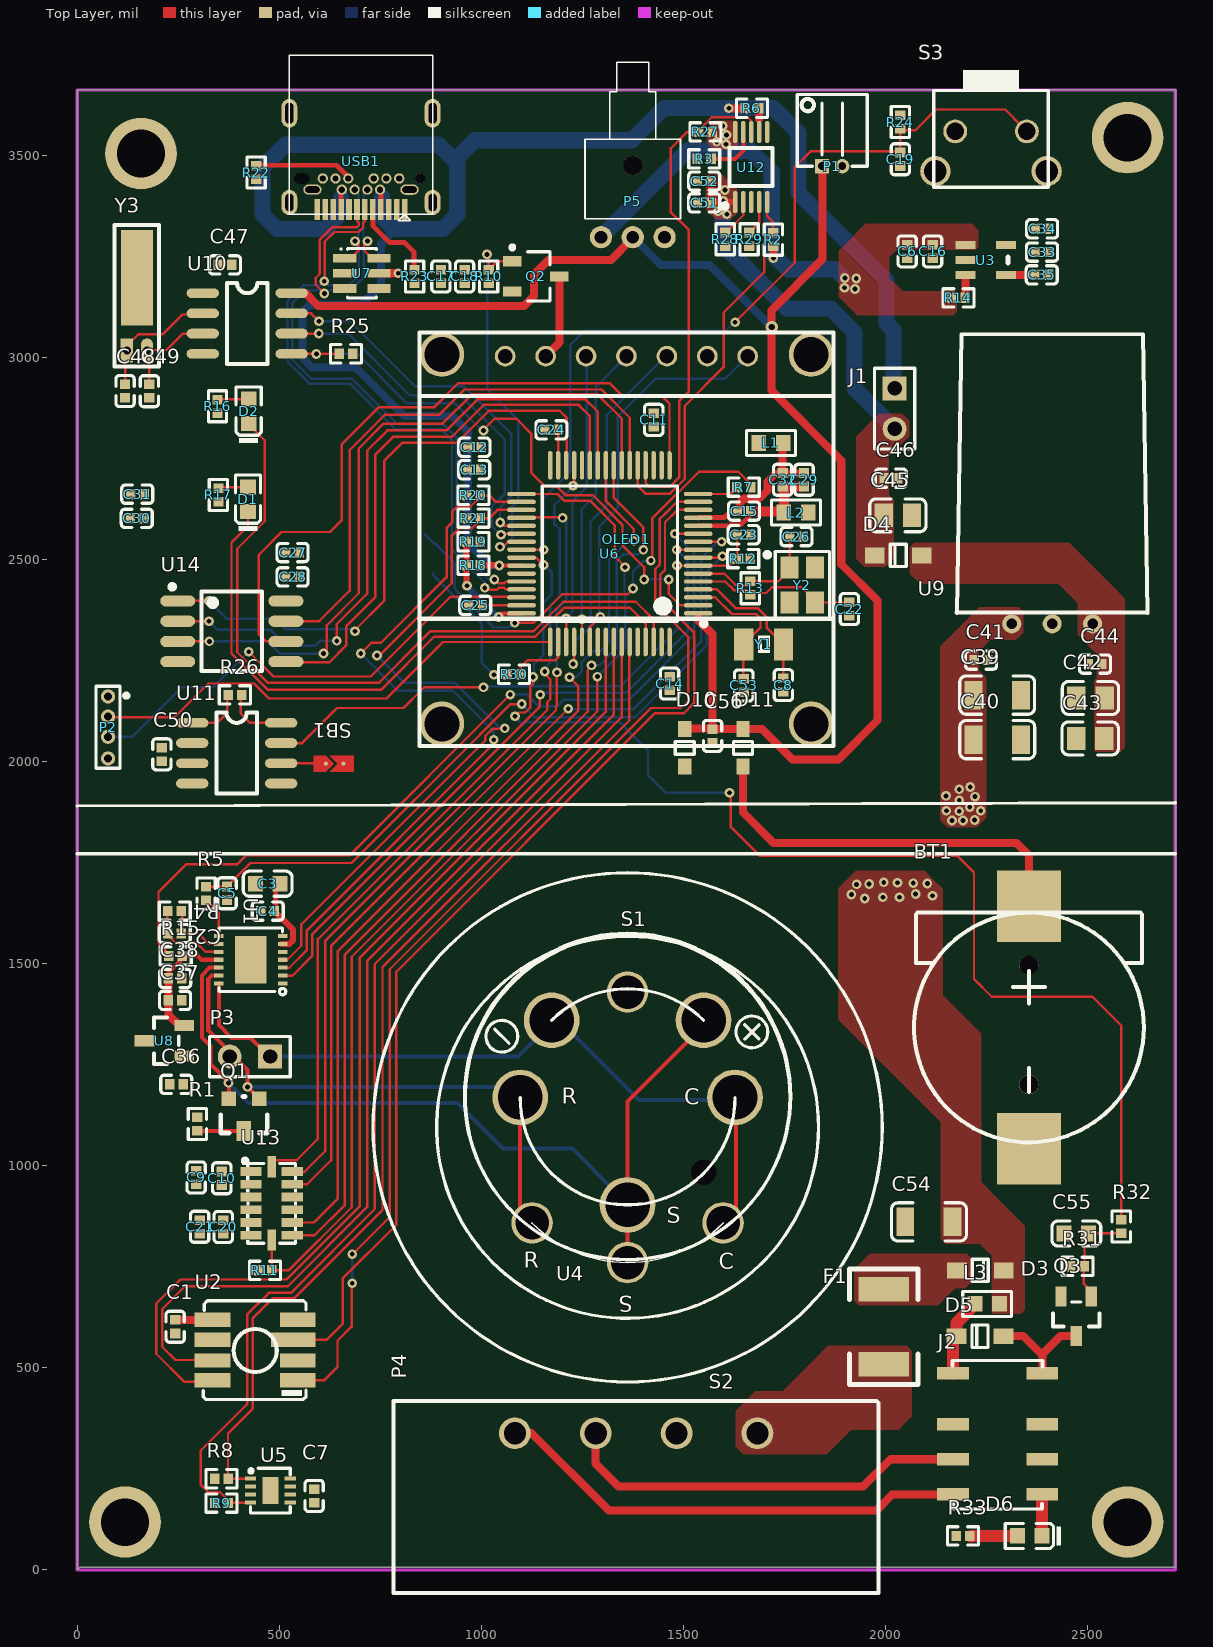
[diagram p0: Top Layer view]
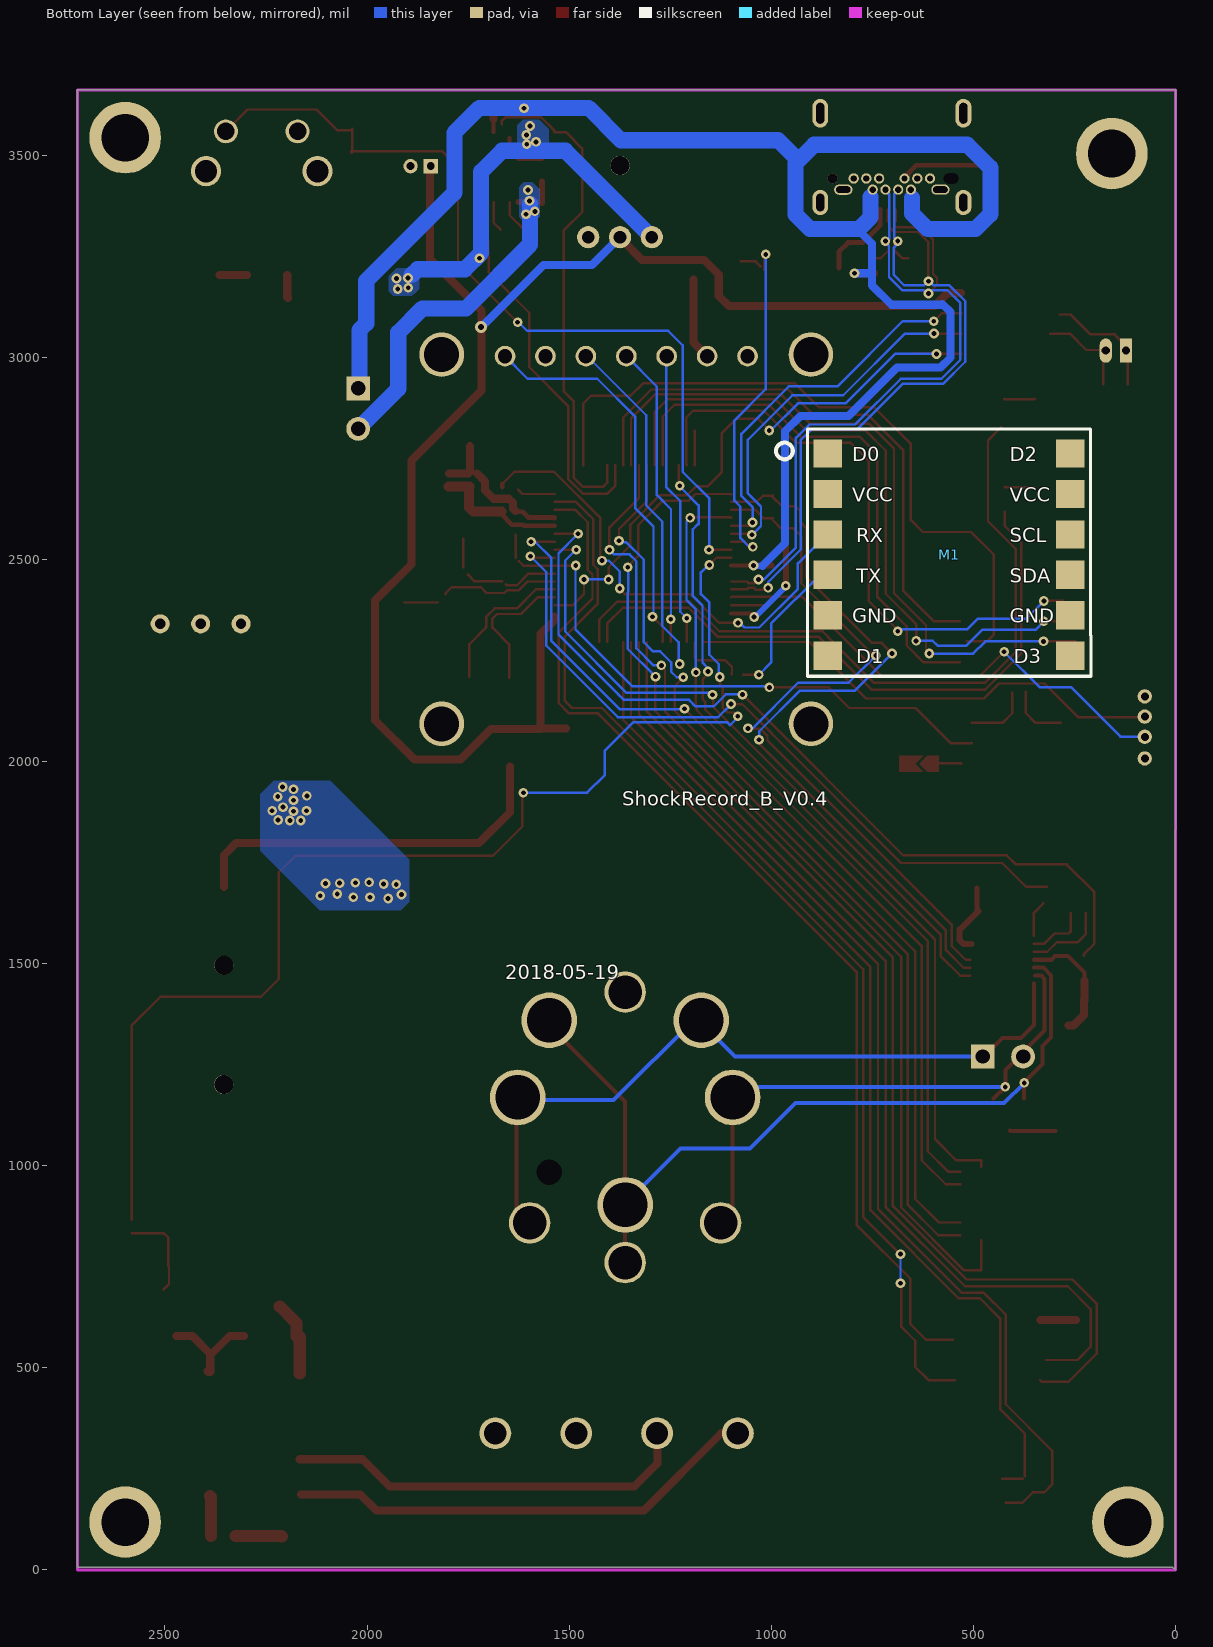
[diagram p1: Bottom Layer view, seen from below]
# Altium PCB MISC105202.PcbDoc (part 1 of 3)
Units mil, origin at the board's own origin, x right, y up, seen from the top; angles counter-clockwise.
Board outline 2717.72 x 3662.2 mil, 4 copper layers (Top Layer, GND, POWER, Bottom Layer), stack 38.217 mil thick; 136 components, 101 nets, 484 pads, 108 vias.
Unrouted connection lines stored in the file: 61.

## Layer stack, top to bottom
Top Layer: signal copper 1.4
Dielectric: core 10, FR-4, Dk 4.2
GND: plane copper 1.417, net GND
Dielectric: prepreg 10, Dk 4.2
POWER: plane copper 1.4, net (Multiple Nets)
Dielectric: core 12.6, FR-4, Dk 4.8
Bottom Layer: signal copper 1.4

## Board outline
0,-0.39 7.09,6.69 2717.32,6.69 2717.32,3661.81 -0.39,3661.81

## Design rules (kind name [scope] priority, off if disabled: settings)
Clearance Clearance_1 [inpolygon] p1: gap=6
Clearance [All] p2: gap=6
DiffPairsRouting [All] p1: maxlimit=6 minlimit=6 mostfreqgap=6 maxuncoupledlength=500
HoleSize [All] p1: absolutevalues=TRUE maxlimit=150 minlimit=10 maxpercent=80.000 minpercent=20.000
MinimumSolderMaskSliver [All] p1: minsoldermaskwidth=0
PlaneClearance [All] p1: clearance=20
PlaneConnect [All] p1: planeconnectstyle=Direct reliefexpansion=20 reliefentries=4 reliefconductorwidth=10 reliefairgap=10
PolygonConnect PolygonConnect_2 [All vs isvia] p1: connectstyle=Direct reliefconductorwidth=10 reliefentries=4 polygonreliefangle="90 Angle"
PolygonConnect PolygonConnect_1 [InNet(gnd)] p2: connectstyle=Relief reliefconductorwidth=15 reliefentries=4 polygonreliefangle="90 Angle"
PolygonConnect [All] p3: connectstyle=Direct reliefconductorwidth=15 reliefentries=4 polygonreliefangle="90 Angle"
RoutingVias [All] p1: holewidth=28 width=50 viastyle="Through Hole" minholewidth=10 minwidth=20 maxholewidth=50 maxwidth=100
SilkToSilkClearance [All] p1: silktosilkclearance=0
SilkscreenOverComponentPads SilkToSolderMaskClearance [IsPad] p1: minsilkscreentomaskgap=0
SolderMaskExpansion [All] p1: expansion=4
Width [All] p1: maxlimit=40 minlimit=6 preferedwidth=6 minimp=50.000000 maximp=50.000000 favimp=50.000000
21 further rules are at their usual default settings.

## Classes and differential pairs
component class ShockRecord_V0.45: C8 C9 C10 C11 C12 C13 C14 C15 C17 C18 C19 C20 C21 C22 C23 C24 C25 C26 C27 C28 C30 C31 C47 C48 C49 C50 C51 C52 C53 D1 D2 M1 OLED1 P1 P2 P5 Q2 R2 R3 R6 R7 R10 R11 R12 R13 R16 R17 R18 R19 R20 R21 R22 R23 R24 R25 R26 R27 R28 R29 R30 S3 SB1 U6 U7 U10 U11 U12 U13 U14 USB1 Y1 Y2 Y3
component class ShockRecord_PWR_V0.45: BT1 C6 C16 C29 C32 C33 C34 C35 C36 C37 C38 C39 C40 C41 C42 C43 C44 C45 C46 C54 C55 C56 D3 D4 D5 D6 D10 D11 F1 J1 J2 L1 L2 L3 P4 Q3 R14 R15 R31 R32 R33 U3 U8 U9
component class ShockRecord_Sensor_V0.45: C1 C2 C3 C4 C5 C7 P3 Q1 R1 R4 R5 R8 R9 S1 S2 U1 U2 U4 U5
differential pair D: +D_P -D_N

## Components (designator, comment, footprint, x,y, rotation, side; value= is the part's Value field where it differs from the comment)
BT1 "CR2032-3V" BT1 2342.52,1322.44 r90 top
C1 "0.1uF,25V" 0402_C 242.13,601.57 r270 top
C2 "1uF (105) 10% 50V" 0402_C 240.94,1574.41 r180 top
C3 "10uF" 0603_C 470.87,1697.64 r0 top
C4 "0.1uF,25V" 0402_C 471,1630 r0 top
C5 "1uF,25V" 0402_C 370.47,1674.02 r90 top
C6 "0.1uF" 0402_C 2053,3262 r270 top
C7 "0.1uF" 0402_C 586,183 r270 top
C8 "2.7pF" 0402_C 1746.85,2188.98 r270 top
C9 "1uF" 0402_C 294.09,970.87 r270 top
C10 "0.1uF" 0402_C 357.48,968.9 r90 top
C11 "0.1uF" 0402_C 1425.98,2845.28 r270 top
C12 "0.1uF" 0402_C 982.28,2777.56 r0 top
C13 "0.1uF" 0402_C 981.89,2721.65 r0 top
C14 "0.1uF" 0402_C 1465.35,2192.91 r90 top
C15 "0.1uF" 0402_C 1649.61,2619.68 r180 top
C16 "10uF" 0402_C 2116,3262 r90 top
C17 "0.1uF" 0402_C 899.61,3200 r270 top
C18 "10uF" 0402_C 958.27,3200 r270 top
C19 "10nF" 0402_C 2036.22,3489.96 r270 top
C20 "1uF" 0402_C 361.02,848.43 r90 top
C21 "0.1uF" 0402_C 302.76,848.82 r270 top
C22 "20pF" 0402_C 1910,2377 r90 top
C23 "0.1uF" 0402_C 1648.82,2561.02 r180 top
C24 "F0.1uF_L0R" 0402_C 1172.83,2820.47 r0 top
C25 "F0.1uF_L0R" 0402_C 984.65,2386.22 r0 top
C26 "20pF" 0402_C 1779.13,2556.3 r180 top
C27 "1uF" 0402_C 532.68,2516.93 r0 top
C28 "0.1uF" 0402_C 532.68,2456.69 r180 top
C29 "100nF,16V" 0402_C 1798,2697 r90 top
C30 "1uF" 0402_C 147.24,2601.57 r180 top
C31 "0.1uF" 0402_C 148.43,2661.42 r0 top
C32 "10uF, 6.3V" 0402_C 1745,2697 r90 top
C33 "100nF,16V" 0402_C 2386.78,3260.44 r180 top
C34 "10uF, 6.3V" 0402_C 2387,3318 r180 top
C35 "0.1uF" 0402_C 2386,3204 r180 top
C36 "10uF, 6.3V" 0402_C 244.88,1201.18 r0 top
C37 "100nF,16V" 0402_C 241.93,1409.06 r180 top
C38 "10uF, 6.3V" 0402_C 242.13,1463.39 r180 top
C39 "10uF,50V" 1206_C 2275.76,2164.28 r180 top
C40 "10uF,50V" 1206_C 2276,2054 r180 top
C41 "0.1uF" 0402_C 2236,2251 r0 top
C42 "22uF,25V" 0805_C 2506.58,2157.18 r0 top
C43 "22uF,25V" 0805_C 2506,2057 r0 top
C44 "0.1uF" 0402_C 2518,2241 r180 top
C45 "22uF,25V" 0805_C 2030,2609 r180 top
C46 "0.1uF" 0402_C 2013,2701 r0 top
C47 "0.1uF" 0402_C 365.16,3228.74 r180 top
C48 "10pF" 0402_C 118.11,2916.54 r270 top
C49 "10pF" 0402_C 178.35,2916.14 r270 top
C50 "0.1uF" 0402_C 209.25,2017.72 r90 top
C51 "10uF" 0402_C 1551,3382 r0 top
C52 "0.1uF" 0402_C 1551,3436 r180 top
C53 "2.7pF" 0402_C 1648.82,2188.19 r270 top
C54 "10uF,50V" 1206_C 2107,861 r0 top
C55 "22uF,6.3V" 0603_C 2471.65,832.28 r0 top
C56 "0.1uF" 0402_C 1571.65,2063.39 r90 top
D1 "Green" 0603_LED_S1 422.28,2648.58 r90 top
D2 "Red" 0603_LED_S1 424.02,2866.14 r90 top
D3 "B5819W  SL" SOD-123 2234,741 r180 top
D4 "B5819W  SL" SOD-123 2031,2510 r0 top
D5 "B5819W  SL" SOD-123 2233,578 r0 top
D6 "Green" 0603_LED_S1 2356,84 r180 top
D10 "1N4148WS T4" SOD-323 1502.76,2033.86 r270 top
D11 "1N4148WS T4" SOD-323 1646.85,2033.86 r270 top
F1 "SMD1812P050TF/30" 1812 1995,694 r270 top
J1 "PSEL" HDR1X2 2022,2923 r270 top
J2 "G6KU-2G-Y" G6KU-2G-Y 2276.94,486.24 r270 top
L1 "10uH ±10%" 0603_L 1716,2788 r180 top
L2 "10uH ±10%" 0603_L 1778,2616 r0 top
L3 "10uH ±10%" 0603_L 2251,658 r180 top
M1 "JY-901" JY-901 860.87,2262.18 r180 bottom locked
OLED1 "OLED-SPI-0.96" OLED_SPI_0.96 1358.66,3002.76 r0 top locked
P1 "BAT" 1.27*2L 1867.52,3472.83 r0 top
P2 "SWD" 127*4 75.98,2161.02 r270 top
P3 "2S" HDR1X2 477,1270 r180 top
P4 "PWR" 508*4B 1382.68,338.19 r0 top
P5 "SW-3" KG 1374.23,3385.73 r180 top
Q1 "J177" SOT-23 450,1166 r180 top
Q2 "AO3401" SOT-23-3L 1134.07,3199.97 r180 top
Q3 "SS8050 Y1" SOT-23(SOT-23-3) 2471.26,627.56 r90 top
R1 "1.1KΩ (1101) ±1%" 0402_R 297,1103 r90 top
R2 "10K" 0402_R 1722,3291 r270 top
R3 "10K" 0402_R 1551,3491 r0 top
R4 "1.1KΩ (1101) ±1%" 0402_R 240.94,1629.92 r180 top
R5 "100R" 0402_R 318.5,1673.62 r90 top
R6 "10K" 0402_R 1669,3616 r180 top
R7 "120Ω" 0402_R 1648.82,2678.74 r0 top
R8 "4.7K" 0402_R 357.09,225.59 r180 top
R9 "4.7K" 0402_R 357.09,165.35 r180 top
R10 "10K" 0402_R 1017.72,3200 r90 top
R11 "10K" 0402_R 464.17,740.94 r180 top
R12 "10K" 0402_R 1647.64,2501.97 r0 top
R13 "1M" 0402_R 1664.96,2428.74 r270 top
R14 "10K" 0402_R 2180,3147 r180 top
R15 "100Ω (1000) ±1%" 0402_R 243.31,1518.9 r180 top
R16 "1K" 0402_R 346.85,2878.74 r270 top
R17 "1K" 0402_R 349.28,2659.58 r270 top
R18 "FDNP_L0R" 0402_R 979.92,2485.43 r0 top
R19 "0R" 0402_R 979.92,2543.7 r180 top
R20 "10K" 0402_R 979.92,2658.66 r180 top
R21 "10K" 0402_R 980.31,2601.97 r180 top
R22 "5K1" 0402_R 442.52,3457.09 r270 top
R23 "5K1" 0402_R 834.25,3200 r90 top
R24 "10K" 0402_R 2036.22,3581.89 r90 top
R25 "10K" 0402_R 664.57,3008.66 r0 top
R26 "0R" 0402_R 389.76,2164.57 r180 top
R27 "10K" 0402_R 1553.94,3557.48 r0 top
R28 "1K" 0402_R 1603,3292 r90 top
R29 "2K" 0402_R 1662,3292 r90 top
R30 "120Ω" 0402_R 1080.71,2215.75 r180 top
R31 "100K" 0402_R 2474.41,750.79 r0 top
R32 "680R" 0402_R 2582.68,849.21 r270 top
R33 "1K" 0402_R 2191,84 r180 top
S1 "4NT" EC-3 1361.42,1168.8 r0 top
S2 "C2H4" EC-3-17MM 1361.42,1094.8 r180 top locked
S3 "F1" Reset_TE 2260.55,3460.47 r180 top
SB1 "JUMPER" "JP2_SMD (Primary)" 634.45,1994.49 r0 top
U1 "LPM91002" WSON-14 429.13,1509.45 r180 top
U2 "MS5803" MS5803 439.97,543.7 r0 top
U3 "SP6205-3.3" SOT23-5 2297.45,3203.19 r90 top
U4 "4OXV" EC-2 1361.42,1171.8 r135 top
U5 "SHT31" SHT31 477.56,196.06 r0 top
U6 "STM32F405RGT6" LC-LQFP-64_10x10x05P 1317.53,2514.18 r90 top locked
U7 "TPD4E001DBVR" SOT23-6 703.94,3207.87 r270 top
U8 "REF3125" SOT-23(SOT-23-3) 215.35,1309.06 r0 top
U9 "ZY7805LS-1000" ZY78xxLS-1000 2411.81,2340.55 r0 top
U10 "DS1302" SO-8 310.38,3158.66 r0 top
U11 "SP706R" SO-8 284.25,2095.64 r0 top
U12 "BQ24090" HVSSOP-10 1667.23,3470.73 r0 top
U13 "ADXL345" ADXL345 480.79,906.69 r0 top
U14 "W25Q128FV-8" SOIC-8_208mil 382.3,2321.99 r270 top
USB1 "USB_TypeC_Receptacle" USB_TYPEC 701.78,3493.36 r180 top
Y1 "FC135" FC-135 1698.03,2289.76 r180 top
Y2 "8MHz" LC-SMD-3225_4P 1793.7,2436.61 r270 top
Y3 "DT-38G06Q-32.768K" 32K 87.44,2976.54 r0 top

## Footprints (in the part's own frame and the unit in brackets; to place one, negate y for a bottom-side part, rotate by r counter-clockwise, add the part's x,y. Pads: shape width x height; smd on the part's side, far side on the other; paste and mask are expansions set on the pad)
1.27*2L [mm]
  rect 0.9x0.9 hole 0.5: 1(-0.635,0)
  round 0.9 hole 0.5: 2(0.635,0)
  silkscreen extent -2.2,0 2.2,4.5
32K [mil]
  rect 30x60 hole 20: 1(35,40)
  oval 30x60 hole 20: 2(85,40)
  rect 78.74x236.22 smd: Y3(60,220)
  silkscreen extent 5,0 115,351
127*4 [mm]
  round 0.9 hole 0.5: 1(0,0) 2(1.27,0) 3(2.54,0) 4(3.9,0)
  silkscreen extent -0.64,-0.75 4.52,1.28
0402_C [mm]
  rect 0.6x0.65 smd mask+0.051: 1(-0.425,0) 2(0.425,0)
  silkscreen extent -0.97,-0.58 0.97,0.58, body extent -0.48,-0.3 0.52,0.3, height 0.2
0402_R [mm]
  rect 0.6x0.65 smd mask+0.051: 1(-0.425,0) 2(0.425,0)
  silkscreen extent -0.97,-0.58 0.97,0.58, body extent -0.57,-0.27 0.58,0.28, height 0.41
508*4B [mm]
  round 2 hole 1.4: 1(7.62,0) 2(2.54,0) 3(-2.54,0) 4(-7.62,0)
  silkscreen extent -15.24,-10.03 15.24,2.03
0603_C [mm]
  rect 0.93x0.98 smd: 1(-0.77,0) 2(0.77,0)
  silkscreen extent -1.53,-0.79 1.54,0.79, body extent -0.8,-0.4 0.8,0.4, height 0.3
0603_L [mm]
  rect 0.93x0.98 smd: 1(-0.77,0) 2(0.77,0)
  silkscreen extent -1.53,-0.79 1.54,0.79, body extent -0.82,-0.41 0.82,0.41, height 0.46
0603_LED_S1 [mm]
  rect 0.93x0.98 smd: A(0.77,0) K(-0.77,0)
  silkscreen extent -1.97,-0.79 1.54,0.79, body extent -0.8,-0.4 0.8,0.4, height 0.6
0805_C [mm]
  rect 1.16x1.47 smd: 1(-0.89,0) 2(0.89,0)
  silkscreen extent -1.77,-1.04 1.77,1.04, body extent -1,-0.62 1,0.63, height 0.77
1206_C [mm]
  rect 1.13x1.8 smd: 1(-1.49,0) 2(1.49,0)
  silkscreen extent -2.36,-1.2 2.35,1.2, body extent -1.6,-0.81 1.6,0.79, height 1
1812 [mil]
  rect 60x125 smd: 1(0,0) 2(185,0)
  silkscreen extent -50,-85 235,85
ADXL345 [mm]
  rect 1.345x0.55 smd: 1(-1.298,2) 2(-1.298,1.2) 3(-1.298,0.4) 4(-1.298,-0.4) 5(-1.298,-1.2) 6(-1.298,-2) 8(1.298,-2) 9(1.298,-1.2) 10(1.298,-0.4) 11(1.298,0.4) 12(1.298,1.2) 13(1.298,2)
  rect 0.55x1.345 smd: 7(0,-2.298) 14(0,2.298)
  silkscreen extent -1.81,-2.52 1.6,2.81
BT1 [mm]
  round 1.2 hole 1.2: 0(-3.089,-0.302) 0(4.404,-0.302)
  rect 4.5x4 smd: 1(8.112,-0.302) 2(-7.128,-0.302)
  silkscreen extent -6.73,-7.52 7.71,6.91
EC-2 [mm]
  round 3.5 hole 2.8: 1(0,-6.75) 2(6.75,0)
  round 1 hole 1.6: 3(-6.75,0)
  silkscreen extent -10.25,-10.25 10.25,10.25
EC-3 [mm]
  round 3.5 hole 2.8: 1(6.75,0) 2(0,-6.75) 3(-6.75,0)
  silkscreen extent -10.2,-10.2 10.2,10.2
EC-3-17MM [mm]
  round 2.6 hole 2.1: 0(0,-8.5) 1(-6,6) 2(0,8.5) 3(6,6)
  silkscreen extent -16,-16 16,16
FC-135 [mm]
  rect 1.2x2 smd: 1(-1.25,0) 2(1.25,0)
  silkscreen extent -0.4,-0.55 0.36,0.55
G6KU-2G-Y [mm]
  rect 0.8x2 smd: 1(0,-2.8) 2(3.2,-2.8) 3(5.4,-2.8) 4(7.6,-2.8) 5(7.6,2.8) 6(5.4,2.8) 7(3.2,2.8) 8(0,2.8)
  silkscreen extent -0.8,-2.84 8.53,2.81
HDR1X2 [mm] "Connector; Header; 2 Position"
  rect 1.5x1.5 hole 0.9: 1(0,0)
  round 1.5 hole 0.9: 2(2.54,0)
  silkscreen extent -1.27,-1.27 3.81,1.27
HVSSOP-10 [mm]
  oval 0.28x1.4 smd mask+0.051: 1(-1,-2.2) 2(-0.5,-2.2) 3(0,-2.2) 4(0.5,-2.2) 5(1,-2.2) 6(1,2.2) 7(0.5,2.2) 8(0,2.2) 9(-0.5,2.2) 10(-1,2.2)
  silkscreen extent -1.8,-2.6 1.33,1.2
"JP2_SMD (Primary)" [mil]
  round 10 smd paste-10 mask+3.94: 1(-19.69,0) 2(23.62,0)
  Top Layer region: -9.84,-19.69 49.21,-19.69 49.21,19.68 -9.84,19.68 9.84,0
  Top Layer region: -19.69,19.68 -49.21,19.68 -49.21,-19.69 -19.69,-19.69 0,0
JY-901 [mil]
  rect 70x70 smd: 1(0.63,499.63) 2(0.63,399.63) 3(0.63,299.63) 4(0.63,199.63) 5(0.63,99.63) 6(0.63,-0.37) 7(600.63,-0.37) 8(600.63,99.63) 9(600.63,199.63) 10(600.63,299.63) 11(600.63,399.63) 12(600.63,499.63)
  silkscreen extent -127,-51 652,561
KG [mm]
  round 1.2 hole 1.2 unplated: 0(0,-2.25)
  round 1.4 hole 0.8: 1(-2,2.25) 2(0,2.25) 3(2,2.25)
  silkscreen extent -3,-8.75 3,1.1
LC-LQFP-64_10x10x05P [mm]
  oval 0.28x1.8 smd mask+0.051: 1(-3.75,-5.55) 2(-3.25,-5.55) 3(-2.75,-5.55) 4(-2.25,-5.55) 5(-1.75,-5.55) 6(-1.25,-5.55) 7(-0.75,-5.55) 8(-0.25,-5.55) 9(0.25,-5.55) 10(0.75,-5.55) 11(1.25,-5.55) 12(1.75,-5.55) 13(2.25,-5.55) 14(2.75,-5.55) 15(3.25,-5.55) 16(3.75,-5.55) 33(3.75,5.55) 34(3.25,5.55) 35(2.75,5.55) 36(2.25,5.55) 37(1.75,5.55) 38(1.25,5.55) 39(0.75,5.55) 40(0.25,5.55) 41(-0.25,5.55) 42(-0.75,5.55) 43(-1.25,5.55) 44(-1.75,5.55) 45(-2.25,5.55) 46(-2.75,5.55) 47(-3.25,5.55) 48(-3.75,5.55)
  oval 1.8x0.28 smd mask+0.051: 17(5.55,-3.75) 18(5.55,-3.25) 19(5.55,-2.75) 20(5.55,-2.25) 21(5.55,-1.75) 22(5.55,-1.25) 23(5.55,-0.75) 24(5.55,-0.25) 25(5.55,0.25) 26(5.55,0.75) 27(5.55,1.25) 28(5.55,1.75) 29(5.55,2.25) 30(5.55,2.75) 31(5.55,3.25) 32(5.55,3.75) 49(-5.55,3.75) 50(-5.55,3.25) 51(-5.55,2.75) 52(-5.55,2.25) 53(-5.55,1.75) 54(-5.55,1.25) 55(-5.55,0.75) 56(-5.55,0.25) 57(-5.55,-0.25) 58(-5.55,-0.75) 59(-5.55,-1.25) 60(-5.55,-1.75) 61(-5.55,-2.25) 62(-5.55,-2.75) 63(-5.55,-3.25) 64(-5.55,-3.75)
  silkscreen extent -4.55,-6.05 4.25,4.25
LC-SMD-3225_4P [mm]
  rect 1.4x1.15 smd: 1(-1.1,-0.8) 2(1.1,-0.8) 3(1.1,0.8) 4(-1.1,0.8)
  silkscreen extent -2.1,-2.35 2.1,1.7, body extent -1.6,-1.25 1.6,1.25, height 0.61
MS5803 [mm]
  rect 2.25x0.9 smd: 1(2.68,-1.9) 2(2.68,-0.65) 4(2.68,1.9) 5(-2.68,1.9) 6(-2.68,0.65) 7(-2.68,-0.65) 8(-2.68,-1.9)
  rect 2.8x0.9 smd: 3(2.405,0.65)
  silkscreen extent -3.26,-3.1 3.2,3.1
OLED_SPI_0.96 [mm]
  round 2.8 hole 2.2: 0(-11.6,-23.1) 0(-11.6,0.1) 0(11.6,-23.1) 0(11.6,0.1)
  round 1.3 hole 0.9: 1(-7.62,0) 2(-5.08,0) 3(-2.54,0) 4(0,0) 5(2.54,0) 6(5.08,0) 7(7.62,0)
  silkscreen extent -13.04,-24.5 13,1.5
Reset_TE [mm]
  round 1.9 hole 1.4: 0(-3.5,0) 0(3.5,0)
  round 1.5 hole 1.1: 1(-2.25,-2.5) 2(2.25,-2.5)
  silkscreen extent -3.6,-6.36 3.61,1.01
SHT31 [mm]
  rect 1x1.7 smd: 0(0,0)
  rect 0.7x0.254 smd: 1(-1.25,0.75) 2(-1.25,0.25) 3(-1.25,-0.25) 4(-1.25,-0.75) 5(1.25,-0.75) 6(1.25,-0.25) 7(1.25,0.25) 8(1.25,0.75)
  silkscreen extent -1.32,-1.4 1.25,1.4
SO-8 [mil]
  oval 80x24 smd: 1(0,0) 2(0,-50) 3(0,-100) 4(0,-150) 5(220,-150) 6(220,-100) 7(220,-50) 8(220,0)
  silkscreen extent 60,-175 160,25
SOD-123 [mm]
  rect 1.25x1 smd: 1(1.475,0) 2(-1.475,0)
  silkscreen extent -0.5,-0.7 0.5,0.7, body extent -1.85,-0.77 1.85,0.78, height 1.35
SOD-323 [mm]
  rect 1x0.83 smd: 1(1.18,0) 2(-1.18,0)
  silkscreen extent -0.4,-0.6 0.4,0.6, body extent -1.35,-0.63 1.35,0.63, height 1.1
SOIC-8_208mil [mm]
  oval 0.7x2.2 smd: 1(-1.905,-3.4) 2(-0.635,-3.4) 3(0.635,-3.4) 4(1.905,-3.4) 5(1.905,3.4) 6(0.635,3.4) 7(-0.635,3.4) 8(-1.905,3.4)
  silkscreen extent -2.95,-3.9 2.5,1.9